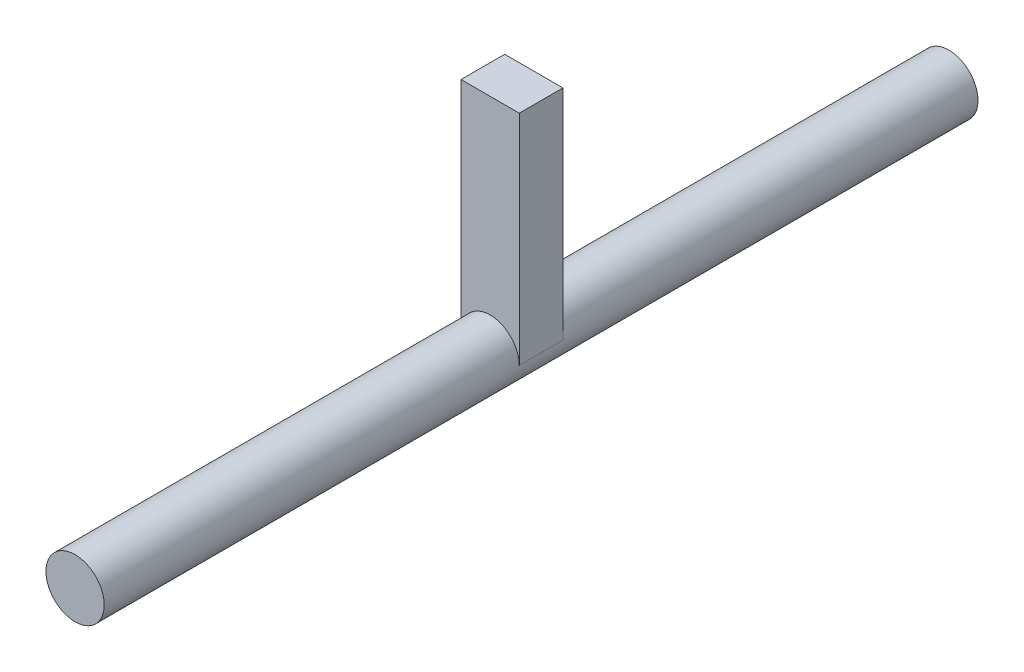
from build123d import *

# Parameters (mm, degrees)
SKETCH1_R           = 4
BOSS_EXTRUDE1_DEPTH = 120
SKETCH2_W           = 8
SKETCH2_H           = 6
BOSS_EXTRUDE2_DEPTH = 30


with BuildPart() as part:
    # Sketch1 → Boss-Extrude1 (new body)
    with BuildSketch(Plane.XY):
        with Locations(Location((0, 0, 0), (0, 0, 180))):
            Circle(SKETCH1_R)
    extrude(amount=BOSS_EXTRUDE1_DEPTH)

    # Sketch2 → Boss-Extrude2 (add)
    with BuildSketch(Plane(origin=(0, 0, 0), x_dir=(1, 0, 0), z_dir=(0, 1, 0))):
        with Locations((0, -60)):
            Rectangle(SKETCH2_W, SKETCH2_H)
    extrude(amount=BOSS_EXTRUDE2_DEPTH)


solid = part.part
